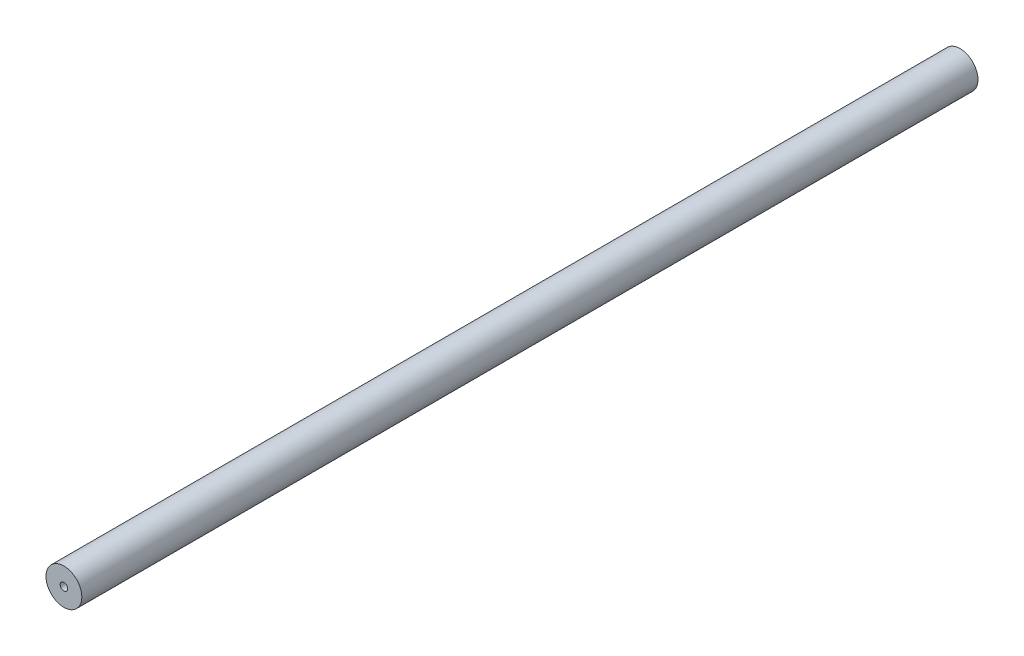
from build123d import *

# Parameters (mm, degrees)
SKETCH_1_R             = 10
EXTRUDE_1_DEPTH        = 500
HOLE_WIZARD_M5_1_D     = 4.2
HOLE_WIZARD_M5_1_DEPTH = 12.4
HOLE_WIZARD_M5_1_TIP   = 1.2618073
HOLE_WIZARD_M5_2_D     = 4.2
HOLE_WIZARD_M5_2_DEPTH = 12.4
HOLE_WIZARD_M5_2_TIP   = 1.2618073


with BuildPart() as part:
    # 草图1 → 凸台-拉伸1 (new body)
    with BuildSketch(Plane.XY):
        Circle(SKETCH_1_R)
    extrude(amount=EXTRUDE_1_DEPTH)

    # M5 螺纹孔1
    with Locations(Plane(origin=(0, 0, 0), x_dir=(-1, 0, 0), z_dir=(0, 0, -1))):
        with Locations((0, 0)):
            Hole(HOLE_WIZARD_M5_1_D / 2, depth=HOLE_WIZARD_M5_1_DEPTH)
            with Locations((0, 0, -(HOLE_WIZARD_M5_1_DEPTH + HOLE_WIZARD_M5_1_TIP / 2))):  # 118° drill point
                Cone(0, HOLE_WIZARD_M5_1_D / 2, HOLE_WIZARD_M5_1_TIP, mode=Mode.SUBTRACT)

    # M5 螺纹孔2
    with Locations(Plane.XY.offset(500)):
        with Locations((0, 0)):
            Hole(HOLE_WIZARD_M5_2_D / 2, depth=HOLE_WIZARD_M5_2_DEPTH)
            with Locations((0, 0, -(HOLE_WIZARD_M5_2_DEPTH + HOLE_WIZARD_M5_2_TIP / 2))):  # 118° drill point
                Cone(0, HOLE_WIZARD_M5_2_D / 2, HOLE_WIZARD_M5_2_TIP, mode=Mode.SUBTRACT)


solid = part.part
